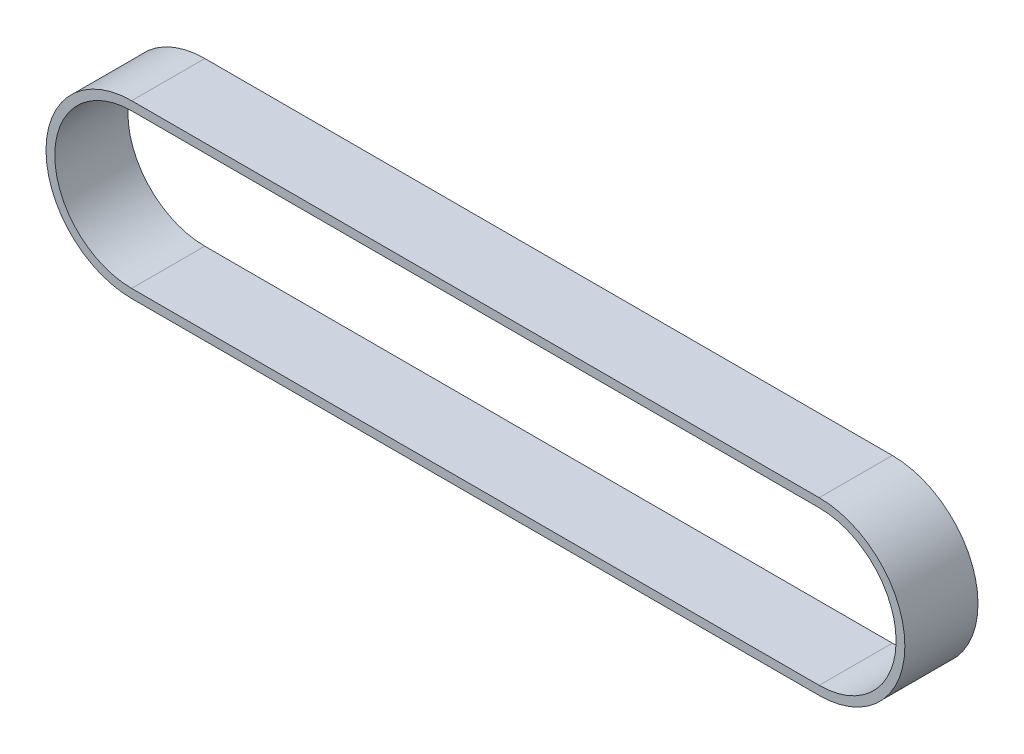
from build123d import *

# Parameters (mm, degrees)
EXTRUDE_THIN1_DEPTH = 12.5


with BuildPart() as part:
    # Sketch2 → Extrude-Thin1 (new, symmetric)
    with BuildSketch(Plane.XY):
        with BuildLine():
            Line((-235, 29.28), (0, 29.28))
            ThreePointArc((0, 29.28), (29.28, 0), (0, -29.28))
            Line((0, -29.28), (-235, -29.28))
            ThreePointArc((-235, -29.28), (-264.28, 0), (-235, 29.28))
        make_face()
        with BuildLine():
            Line((-235, 26.28), (0, 26.28))
            ThreePointArc((0, 26.28), (26.28, 0), (0, -26.28))
            Line((0, -26.28), (-235, -26.28))
            ThreePointArc((-235, -26.28), (-261.28, 0), (-235, 26.28))
        make_face(mode=Mode.SUBTRACT)
    extrude(amount=EXTRUDE_THIN1_DEPTH, both=True)


solid = part.part
